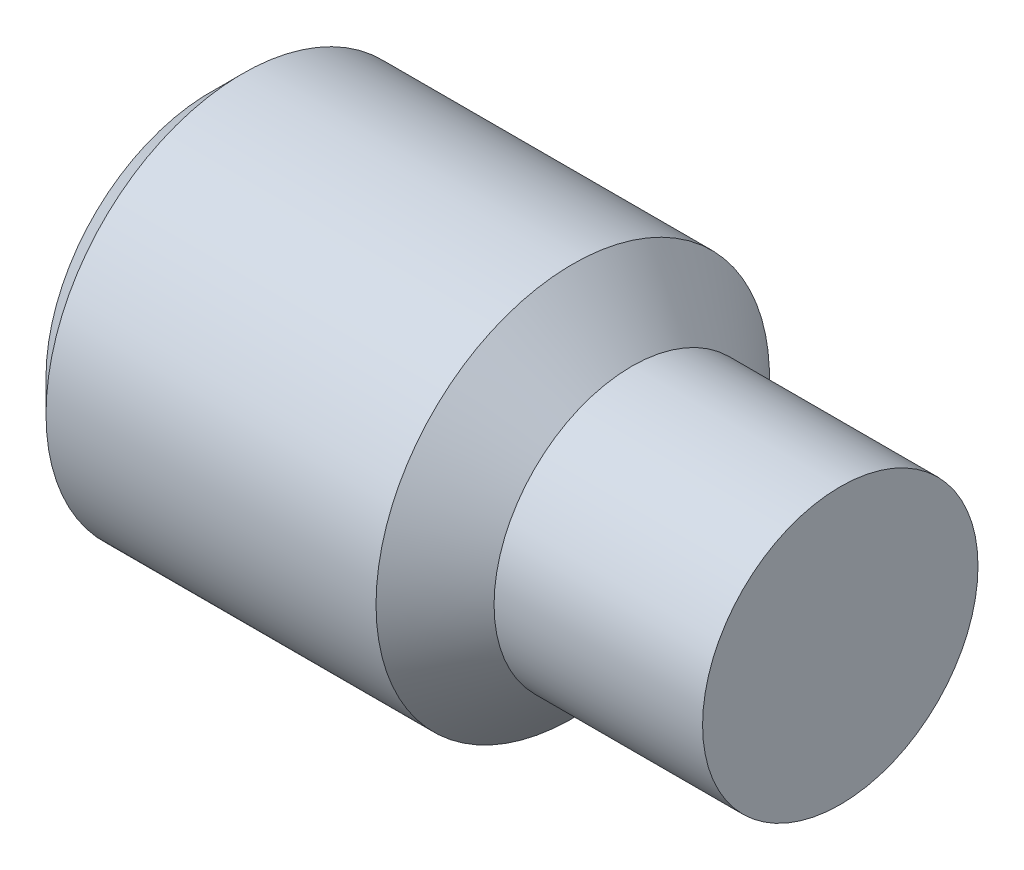
SolidWorks part; units mm, degrees
ref_plane "Front" through (0, 0, 0) normal (0, 0, 1) x (1, 0, 0)
ref_plane "Top" through (0, 0, 0) normal (0, 1, 0) x (1, 0, 0)
ref_plane "Right" through (0, 0, 0) normal (1, 0, 0) x (0, 0, -1)
other "Configuration Table"
sketch "Sketch1" plane through (0, 0, 0) normal (0, 0, 1) x (1, 0, 0)
  line L0 (0, 0) -> (16, 0)
  line L1 (16, 0) -> (16, 3.5)
  line L2 (9.2, 5) -> (10.7, 3.5)
  line L3 (9.2, 5) -> (0.812, 5)
  line L4 (0.812, 5) -> (0, 4.188)
  line L5 (0, 4.188) -> (0, 0)
  line L6 (-1.9688, 0) -> (10.951, 0) construction
  line L7 (16, 3.5) -> (10.7, 3.5)
revolve "Base" add sketch "Sketch1" angle 360 about L6
cosmetic thread "ThreadCosmetic1" [suppressed] parameters "D2"=8.376
sketch "Sketch2" plane through (0, -1.1285, -0.3504) normal (-1, 0, 0) x (0, 0, 1)
  line L1 (3.2371, 1.1285) -> (1.7937, 3.6285)
  line L2 (1.7937, 3.6285) -> (-1.093, 3.6285)
  line L3 (-1.093, 3.6285) -> (-2.5364, 1.1285)
  line L4 (-2.5364, 1.1285) -> (-1.093, -1.3715)
  line L5 (-1.093, -1.3715) -> (1.7937, -1.3715)
  line L6 (1.7937, -1.3715) -> (3.2371, 1.1285)
  circle A0 centre (0.3504, 1.1285) radius 2.5 construction
  dimension "s" = 5
  dimension "e" = 5.7735
extrude "HexagonSocket" cut sketch "Sketch2" against normal blind 4
sketch "Sketch3" plane through (0, 0, 0) normal (0, 0, 1) x (1, 0, 0)
  line L0 (4, 2.5) -> (4, 0)
  line L1 (4, 0) -> (4.8, 0)
  line L3 (4.8, 0) -> (4, 2.5)
  line L4 (-0.331, 0) -> (6.7238, 0) construction
revolve "Cut-Revolve1" cut sketch "Sketch3" angle 360 about L4
sketch "Sketch4" plane through (0, 0, 0) normal (0, 0, 1) x (1, 0, 0)
  line L0 (0.812, 4.2968) -> (1.218, 5)
  line L1 (1.218, 5) -> (1.218, 5.812)
  line L2 (1.218, 5.812) -> (0.406, 5.812)
  line L3 (0.406, 5.812) -> (0.406, 5)
  line L4 (0.406, 5) -> (0.812, 4.2968)
  line L5 (0, 0) -> (2.4831, 0) construction
  line L6 (0.812, 5) -> (0.812, -5) construction
revolve "Cut-Revolve10" [suppressed] cut sketch "Sketch4" angle 360 about L5
pattern_linear "LPattern10" [suppressed] count 10 spacing 0.9744 along (1, 0, 0)
equation "\"df@Sketch1\" = \"D2@ThreadCosmetic1\""
equation "\"h@Sketch3\" = 0.2 * \"t@HexagonSocket\""
equation "\"D1@Sketch4\" = \"d@Sketch1\""
equation "\"D2@Sketch4\" =  ( \"d@Sketch1\" - \"D2@ThreadCosmetic1\" )  / 2"
equation "\"D3@LPattern10\" = \"D2@Sketch4\" * 1.2"
equation "\"D1@LPattern10\" =  ( \"l@Sketch1\" - \"z@Sketch1\" -  ( \"d@Sketch1\" - \"df@Sketch1\" )  / 2 )  / \"D3@LPattern10\""
